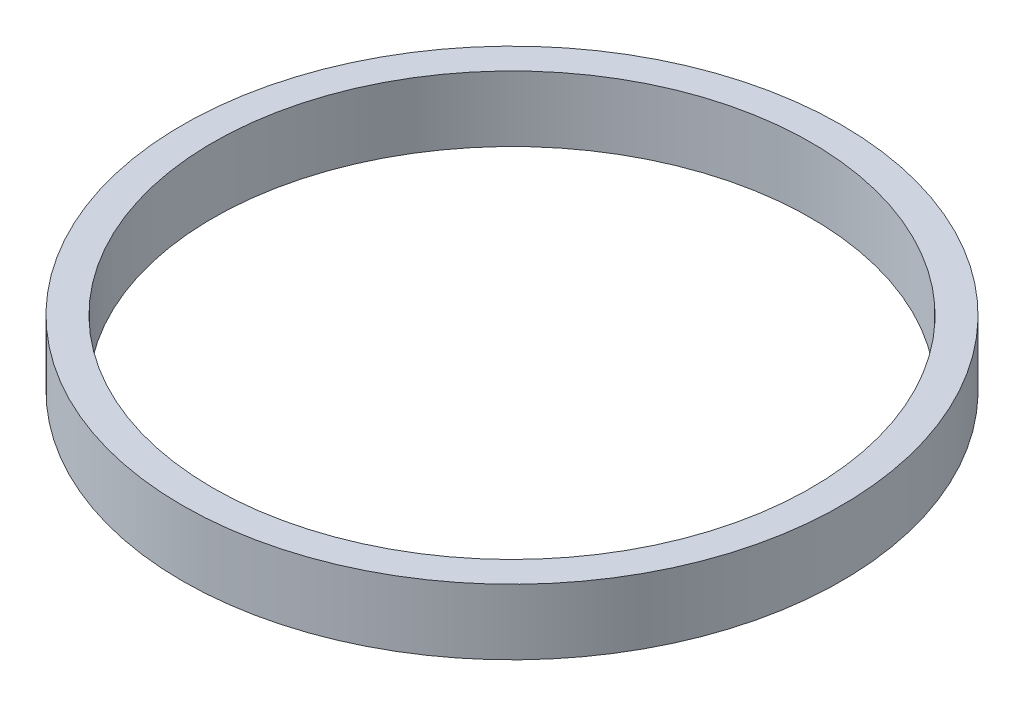
from build123d import *

# Parameters (mm, degrees)
SKETCH1_W = 6.5
SKETCH1_H = 14


with BuildPart() as part:
    # Sketch1 → Revolve1 (revolve)
    with BuildSketch(Plane.XY, mode=Mode.PRIVATE) as revolve1_sk:
        with Locations((67.245706961, 144.5)):
            Rectangle(SKETCH1_W, SKETCH1_H)
    revolve(revolve1_sk.sketch.rotate(Axis((0, 0, 0), (0, -1, 0)), 90), axis=Axis((0, 0, 0), (0, -1, 0)))


solid = part.part
